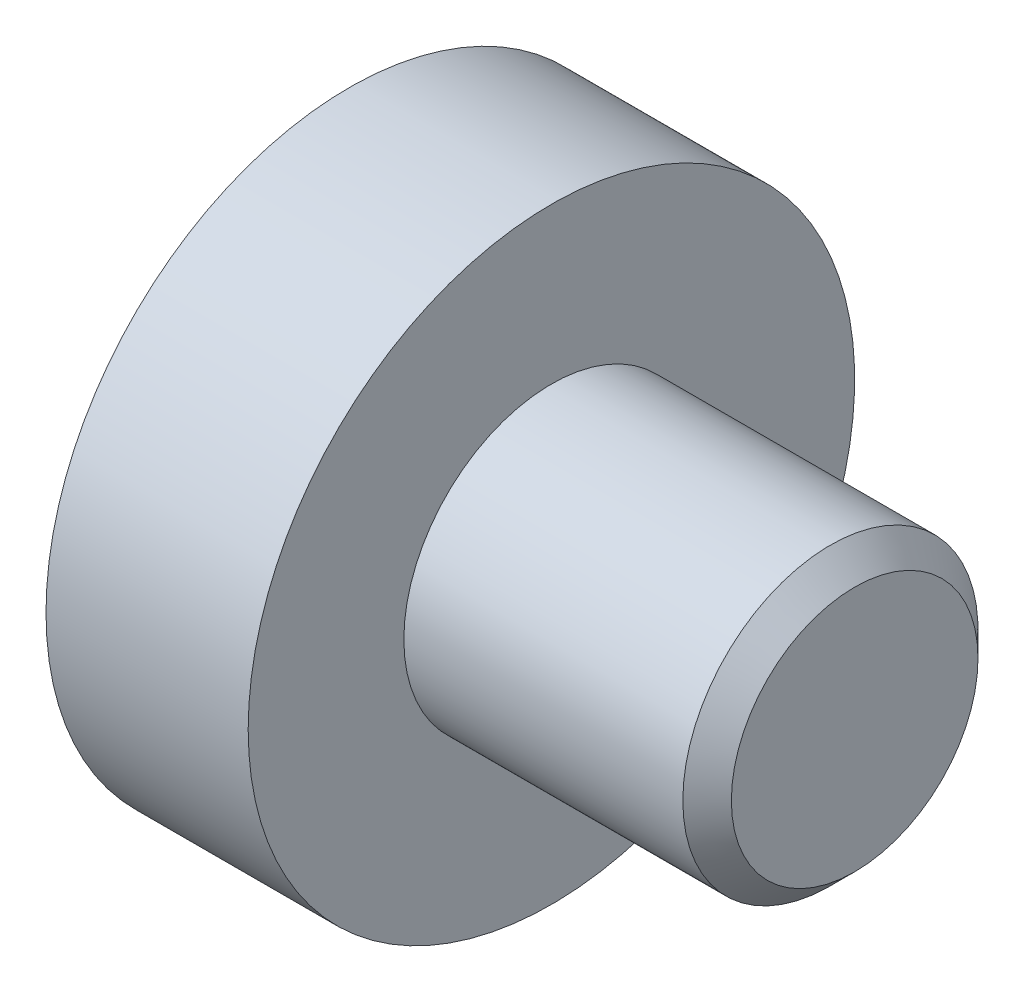
from build123d import *


with BuildPart() as part:
    # Sketch1 → Revolve1 (revolve)
    with BuildSketch(Plane.XY, mode=Mode.PRIVATE) as revolve1_sk:
        Polygon((0, 0), (0, 19.05), (12.7, 19.05), (12.7, 9.271), (30.226, 9.271), (31.75, 7.747), (31.75, 0), align=None)
    revolve(revolve1_sk.sketch.rotate(Axis((-38.775045045, 0, 0), (1, 0, 0)), 90), axis=Axis((-38.775045045, 0, 0), (1, 0, 0)))


solid = part.part
